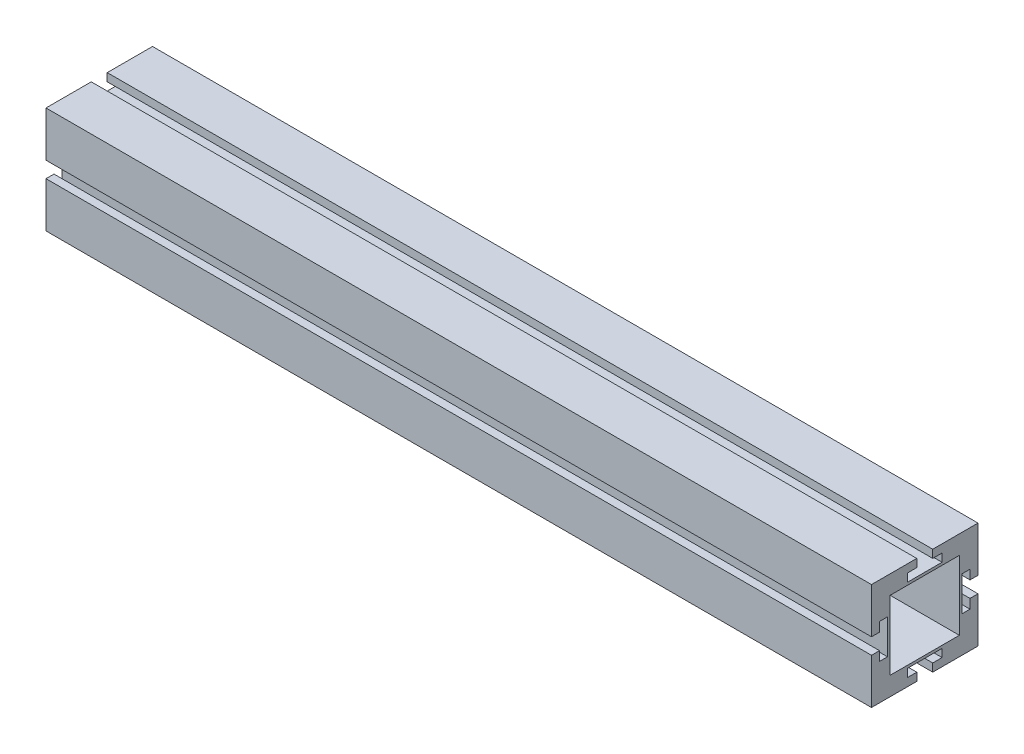
from build123d import *

# Parameters (mm, degrees)
SKETCH1_W           = 26
SKETCH1_H           = 26
BOSS_EXTRUDE1_DEPTH = 310


with BuildPart() as part:
    # Sketch1 → Boss-Extrude1 (new body)
    with BuildSketch(Plane(origin=(0, 0, 0), x_dir=(0, 0, -1), z_dir=(1, 0, 0))):
        Polygon((-20, -20), (-3, -20), (-3, -17), (-6.5, -17), (-6.5, -14), (6.5, -14), (6.5, -17), (3, -17), (3, -20), (20, -20), (20, -3), (17, -3), (17, -6.5), (14, -6.5), (14, 6.5), (17, 6.5), (17, 3), (20, 3), (20, 20), (3, 20), (3, 17), (6.5, 17), (6.5, 14), (-6.5, 14), (-6.5, 17), (-3, 17), (-3, 20), (-20, 20), (-20, 3), (-17, 3), (-17, 6.5), (-14, 6.5), (-14, -6.5), (-17, -6.5), (-17, -3), (-20, -3), align=None)
        Rectangle(SKETCH1_W, SKETCH1_H, mode=Mode.SUBTRACT)
    extrude(amount=BOSS_EXTRUDE1_DEPTH)


solid = part.part
